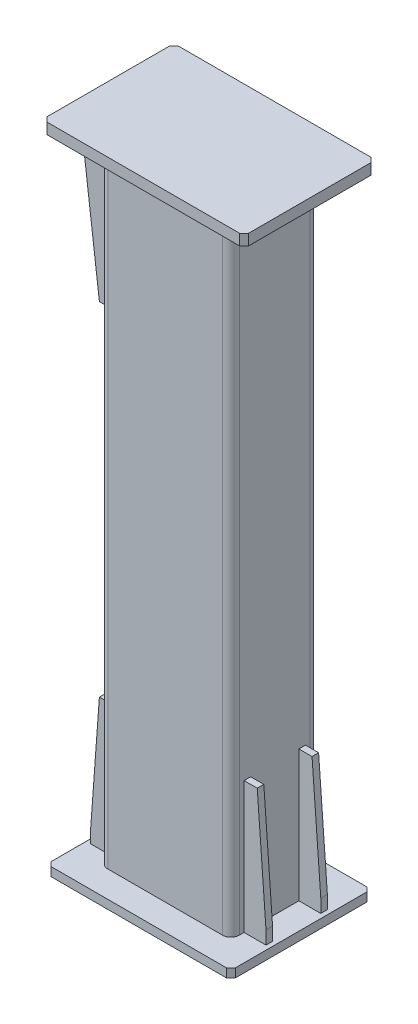
from build123d import *

# Parameters (mm, degrees)
BOSS_EXTRUDE1_DEPTH = 20
BOSS_EXTRUDE2_DEPTH = 1431
BOSS_EXTRUDE3_DEPTH = 25
BOSS_EXTRUDE4_START = -30
BOSS_EXTRUDE4_DEPTH = 15
BOSS_EXTRUDE7_START = -30
BOSS_EXTRUDE7_DEPTH = 15


with BuildPart() as part:
    # Sketch1 → Boss-Extrude1 (new body)
    with BuildSketch(Plane(origin=(0, 0, 0), x_dir=(1, 0, 0), z_dir=(0, 1, 0))):
        Polygon((0, 310), (10, 320), (410, 320), (420, 310), (420, 10), (410, 0), (10, 0), (0, 10), align=None)
    extrude(amount=BOSS_EXTRUDE1_DEPTH)

    # Sketch2 → Boss-Extrude2 (add)
    with BuildSketch(Plane(origin=(0, 20, 0), x_dir=(1, 0, 0), z_dir=(0, 1, 0))):
        with BuildLine():
            Line((79.070897456, 260), (340.929102544, 260))
            ThreePointArc((340.929102544, 260), (354.414263459, 254.414263459), (360, 240.929102544))
            Line((360, 240.929102544), (360, 79.070897456))
            ThreePointArc((360, 79.070897456), (354.414263459, 65.585736541), (340.929102544, 60))
            Line((340.929102544, 60), (79.070897456, 60))
            ThreePointArc((79.070897456, 60), (65.585736541, 65.585736541), (60, 79.070897456))
            Line((60, 79.070897456), (60, 240.929102544))
            ThreePointArc((60, 240.929102544), (65.585736541, 254.414263459), (79.070897456, 260))
        make_face()
        with BuildLine():
            Line((79.070897456, 252), (340.929102544, 252))
            ThreePointArc((340.929102544, 252), (348.757409209, 248.757409209), (352, 240.929102544))
            Line((352, 240.929102544), (352, 79.070897456))
            ThreePointArc((352, 79.070897456), (348.757409209, 71.242590791), (340.929102544, 68))
            Line((340.929102544, 68), (79.070897456, 68))
            ThreePointArc((79.070897456, 68), (71.242590791, 71.242590791), (68, 79.070897456))
            Line((68, 79.070897456), (68, 240.929102544))
            ThreePointArc((68, 240.929102544), (71.242590791, 248.757409209), (79.070897456, 252))
        make_face(mode=Mode.SUBTRACT)
    extrude(amount=BOSS_EXTRUDE2_DEPTH)

    # Sketch3 → Boss-Extrude3 (add)
    with BuildSketch(Plane(origin=(0, 1451, 0), x_dir=(1, 0, 0), z_dir=(0, 1, 0))):
        Polygon((-10, 310), (430, 310), (440, 300), (440, 20), (430, 10), (-10, 10), (-20, 20), (-20, 300), align=None)
    extrude(amount=BOSS_EXTRUDE3_DEPTH)

    # Sketch4 → Boss-Extrude4 (add)
    with BuildSketch(Plane(origin=(0, 0, -260), x_dir=(-1, 0, 0), z_dir=(0, 0, -1)).offset(BOSS_EXTRUDE4_START)):
        Polygon((-30, 320), (-10, 50), (-10, 20), (-410, 20), (-410, 50), (-390, 320), align=None)
    boss_extrude4 = extrude(amount=-BOSS_EXTRUDE4_DEPTH)

    # Mirror1: Boss-Extrude4 across plane
    add(boss_extrude4.mirror(Plane.XY.offset(-160)))

    # Sketch5 → Boss-Extrude7 (add)
    with BuildSketch(Plane.XY.offset(-60).offset(BOSS_EXTRUDE7_START)):
        Polygon((60, 1441), (50, 1451), (-10, 1451), (-10, 1421), (30, 1101), (60, 1101), align=None)
    boss_extrude7 = extrude(amount=-BOSS_EXTRUDE7_DEPTH)

    # Mirror5: Boss-Extrude7 across plane
    add(boss_extrude7.mirror(Plane.XY.offset(-160)))


solid = part.part
